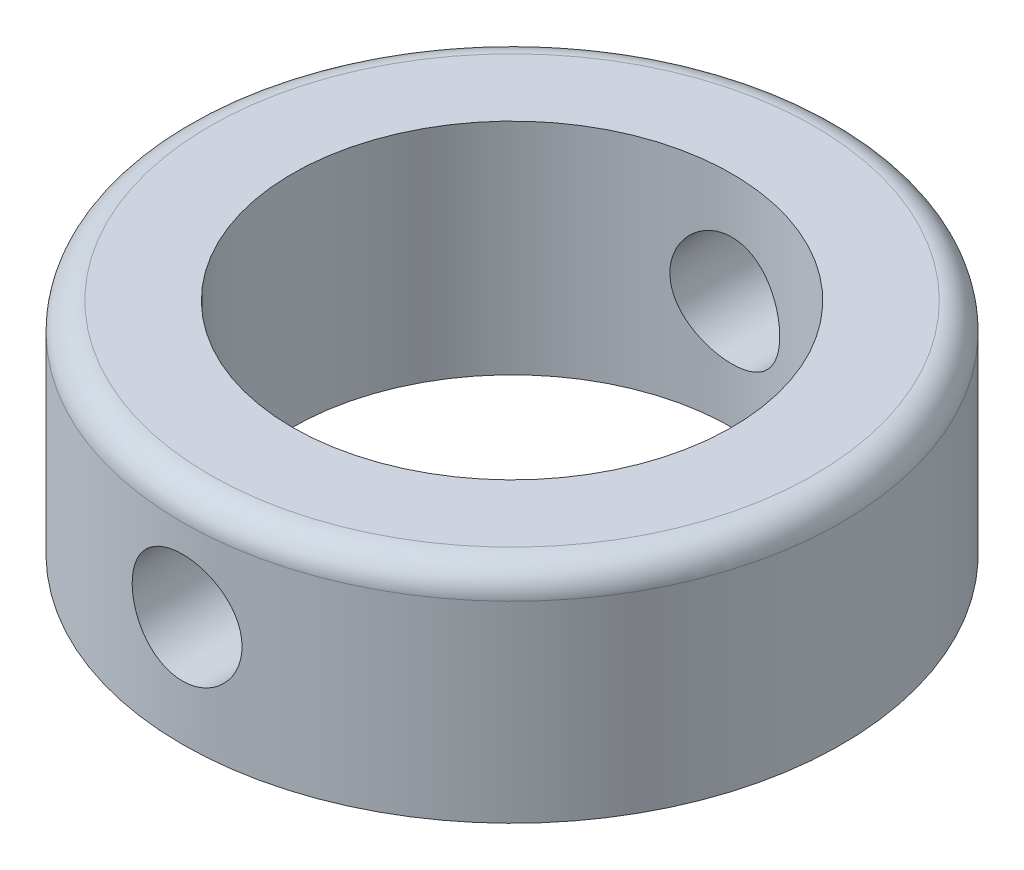
SolidWorks part; units mm, degrees
ref_plane "Front Plane" through (0, 0, 0) normal (0, 0, 1) x (1, 0, 0)
ref_plane "Top Plane" through (0, 0, 0) normal (0, 1, 0) x (1, 0, 0)
ref_plane "Right Plane" through (0, 0, 0) normal (1, 0, 0) x (0, 0, -1)
sketch "Sketch1" plane through (0, 0, 0) normal (0, 1, 0) x (1, 0, 0)
  circle A0 centre (0, 0) radius 12
  circle A1 centre (0, 0) radius 8
  dimension "D1" = 24
  dimension "D2" = 16
extrude "Boss-Extrude1" add sketch "Sketch1" against normal blind 8
sketch "Sketch2" plane through (0, 0, 0) normal (0, 0, 1) x (1, 0, 0)
  line L0 (-12, -8) -> (12, -8) construction
  circle A0 centre (0, -4) radius 2
  point P4 (0, 0)
  dimension "D1" = 4
  dimension "D2" = 4
extrude "Cut-Extrude1" cut sketch "Sketch2" against normal through all both and the other way through all
fillet "Fillet1" radius 1 1 edges at (0, 0, 12)
